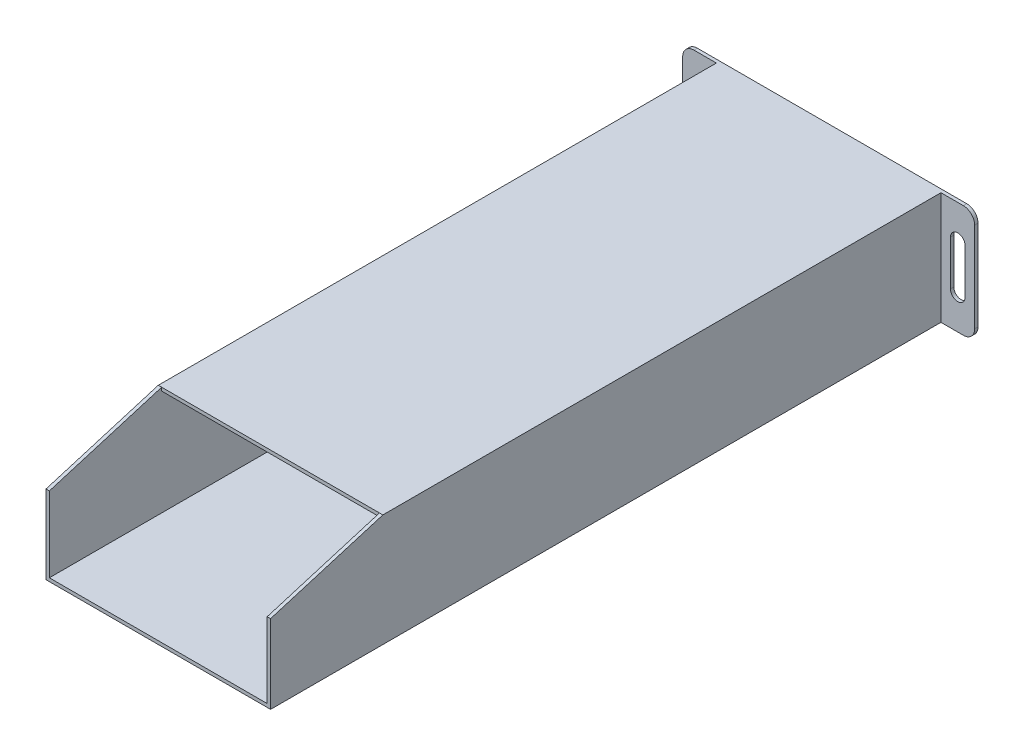
SolidWorks part; units mm, degrees
material "SUS304"
ref_plane "前视基准面" through (0, 0, 0) normal (0, 0, 1) x (1, 0, 0)
ref_plane "上视基准面" through (0, 0, 0) normal (0, 1, 0) x (1, 0, 0)
ref_plane "右视基准面" through (0, 0, 0) normal (1, 0, 0) x (0, 0, -1)
sketch "草图1" plane through (0, 0, 0) normal (0, 0, 1) x (1, 0, 0)
  line L1 (-50, 25) -> (50, 25)
  line L2 (-50, 25) -> (-50, -25)
  line L3 (-50, -25) -> (50, -25)
  line L4 (50, 25) -> (50, -25)
  line L5 (-50, 25) -> (50, -25) construction
  line L6 (-50, -25) -> (50, 25) construction
  point P0 (0, 0)
  dimension "D1" = 100
  dimension "D2" = 50
sketch "草图14" plane through (0, 0, 0) normal (0, 0, 1) x (1, 0, 0)
  line L1 (-50, 25) -> (50, 25)
  line L2 (-50, 25) -> (-50, -25)
  line L3 (-50, -25) -> (50, -25)
  line L4 (50, 25) -> (50, -25)
  line L5 (-50, 25) -> (50, -25) construction
  line L6 (-50, -25) -> (50, 25) construction
  point P0 (0, 0)
  dimension "D1" = 100
  dimension "D2" = 50
extrude "凸台-拉伸1" add sketch "草图14" along normal blind 300
shell "抽壳1" thickness 1.5
sketch "草图15" plane through (0, 0, 0) normal (0, 0, -1) x (-1, 0, 0)
  line L0 (-50, 25) -> (-65, 25)
  line L1 (65, -25) -> (50, -25)
  line L2 (65, -25) -> (65, 25)
  line L3 (65, 25) -> (50, 25)
  line L4 (-65, -25) -> (-65, 25)
  line L5 (65, -25) -> (-65, 25) construction
  line L6 (65, 25) -> (-65, -25) construction
  line L8 (50, -25) -> (50, 25)
  line L9 (-50, -25) -> (-65, -25)
  line L10 (-50, -25) -> (-50, 25)
  line L11 (50, -25) -> (-50, 25) construction
  line L12 (50, 25) -> (-50, -25) construction
  point P0 (0, 0)
  point P6 (0, 0)
  dimension "D1" = 15
extrude "凸台-拉伸2" add sketch "草图15" against normal blind 1.5
sketch "草图16" plane through (50, 0, 0) normal (1, 0, 0) x (0, 0, -1)
  line L0 (-300, 10) -> (-250, 25)
  line L1 (-300, -25) -> (-300, 25) construction
  line L2 (-300, 25) -> (-1.5, 25) construction
  line L3 (-250, 25) -> (-300, 25)
  line L4 (-300, 25) -> (-300, 10)
  dimension "D1" = 15
  dimension "D2" = 50
extrude "切除-拉伸1" cut sketch "草图16" against normal through all
fillet "圆角1" radius 5 4 edges at (65, -25, 0.75) (65, 25, 0.75) (-65, -25, 0.75) (-65, 25, 0.75)
sketch "草图20" plane through (0, 0, 1.5) normal (0, 0, 1) x (1, 0, 0)
  line L0 (-57.5, 25) -> (-57.5, -25) construction
  line L1 (-60, 25) -> (-50, 25) construction
  line L2 (-50, -25) -> (-60, -25) construction
  line L3 (-50, 25) -> (-50, -25) construction
  line L4 (-65, 0) -> (-50, 0) construction
  line L5 (-65, -20) -> (-65, 20) construction
  line L6 (-57.5, -10) -> (-57.5, 10) construction
  line L7 (-60.75, -10) -> (-60.75, 10)
  line L8 (-54.25, -10) -> (-54.25, 10)
  arc A0 (-60.75, -10) -> (-54.25, -10) centre (-57.5, -10) ccw
  arc A1 (-54.25, 10) -> (-60.75, 10) centre (-57.5, 10) ccw
  point P14 (-57.5, 0)
  dimension "D3" = 3.25
  dimension "D1" = 7.5
  dimension "D2" = 20
extrude "切除-拉伸4" cut sketch "草图20" against normal through all
mirror "镜向1" about plane through (0, 0, 0) normal (1, 0, 0) of "切除-拉伸4"
sketch "草图21" plane through (0, 25, 0) normal (0, 1, 0) x (1, 0, 0)
  line L1 (-50, -250) -> (50, -250) construction
  line L2 (-48.5, -250) -> (48.5, -250)
  line L3 (-48.5, -250) -> (-48.5, -260)
  line L4 (-48.5, -260) -> (48.5, -260)
  line L5 (48.5, -250) -> (48.5, -260)
  line L6 (48.5, -255) -> (48.5, -300) construction
  dimension "D1" = 10
extrude "切除-拉伸5" cut sketch "草图21" against normal up to next
sketch "折弯-线1" plane through (0, 0, 0) normal (0, 1, 0) x (1, 0, 0)
sketch "边界框1" plane through (0, 0, 0) normal (0, 1, 0) x (1, 0, 0)
